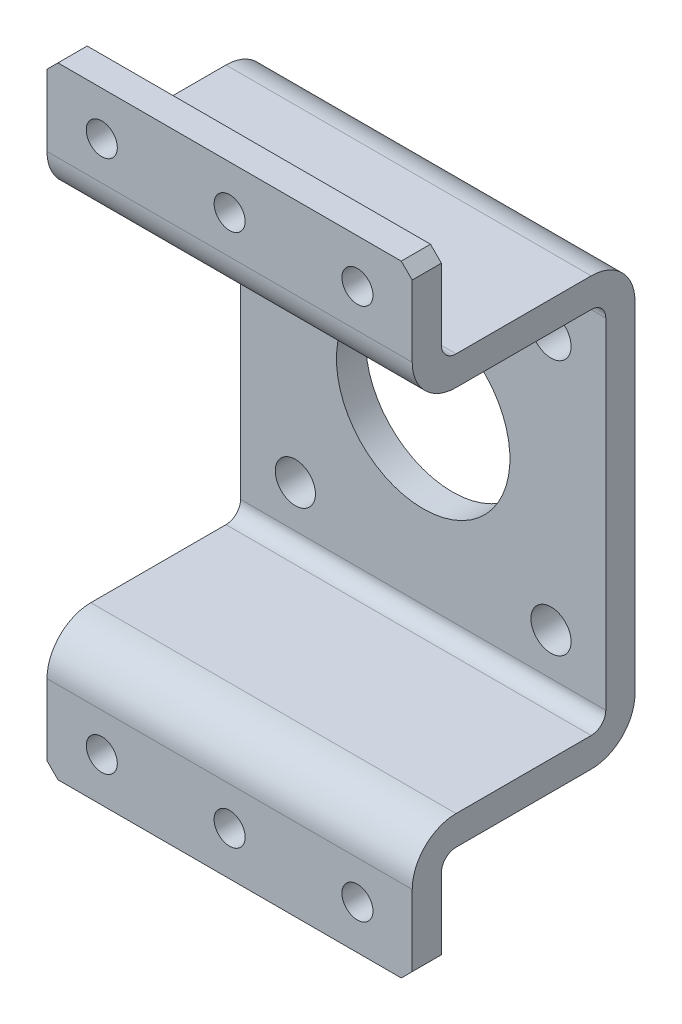
SolidWorks part; units mm, degrees
ref_plane "前视基准面" through (0, 0, 0) normal (0, 0, 1) x (1, 0, 0)
ref_plane "上视基准面" through (0, 0, 0) normal (0, 1, 0) x (1, 0, 0)
ref_plane "右视基准面" through (0, 0, 0) normal (1, 0, 0) x (0, 0, -1)
sketch "草图1" plane through (0, 0, 0) normal (1, 0, 0) x (0, 0, -1)
  line L0 (-61, 85) -> (-61, 50.5)
  line L1 (-53, 85) -> (-53, 58.5)
  line L2 (-53, 58.5) -> (0, 58.5)
  line L3 (0, 58.5) -> (0, -58.5)
  line L4 (0, -58.5) -> (-53, -58.5)
  line L5 (-53, -58.5) -> (-53, -85)
  line L6 (-61, 50.5) -> (-8, 50.5)
  line L7 (-8, 50.5) -> (-8, -50.5)
  line L8 (-8, -50.5) -> (-61, -50.5)
  line L9 (-61, -50.5) -> (-61, -85)
  line L10 (-61, 85) -> (-53, 85)
  line L11 (-61, -85) -> (-53, -85)
  line L12 (0, 0) -> (-67.8043, 0) construction
  point P2 (0, 0)
  dimension "D1" = 8
  dimension "D2" = 61
  dimension "D3" = 117
  dimension "D4" = 170
extrude "凸台-拉伸1" add sketch "草图1" along normal mid plane 100
sketch "草图3" plane through (0, 0, 0) normal (0, 0, -1) x (-1, 0, 0)
  circle A0 centre (0, 0) radius 23.75
  dimension "D1" = 47.5
extrude "切除-拉伸1" cut sketch "草图3" against normal through all
hole_wizard "Ø11.0 (11) 直径孔1" positions "草图5" profile "草图4" hole size "Ø11.0" standard "ISO" end condition through all
sketch "草图5" plane through (0, 0, 0) normal (0, 0, -1) x (-1, 0, 0)
  line L1 (-35, 35) -> (35, 35) construction
  line L2 (-35, 35) -> (-35, -35) construction
  line L3 (-35, -35) -> (35, -35) construction
  line L4 (35, 35) -> (35, -35) construction
  line L5 (-35, 35) -> (35, -35) construction
  line L6 (-35, -35) -> (35, 35) construction
  point P1 (0, 0)
  point P2 (35, -35)
  point P61 (-35, 35)
  point P62 (-35, -35)
  point P63 (35, 35)
  dimension "D1" = 70
  dimension "D2" = 70
sketch "草图4" plane through (0, 0, 0) normal (1, 0, 0) x (0, 1, 0)
  line L0 (0, 0) -> (0, 61)
  line L1 (0, 61) -> (5.5, 61)
  line L2 (5.5, 61) -> (5.5, 0)
  line L5 (5.5, 0) -> (0, 0)
  line L11 (0, -6.35) -> (0, 107.95) construction
  dimension "通孔孔直径" = 11
  dimension "通孔孔深度" = 61
hole_wizard "Ø8.5 (8.5) 直径孔1" positions "草图7" profile "草图6" hole size "Ø8.5" standard "ISO" end condition through all
sketch "草图7" plane through (0, 0, 53) normal (0, 0, -1) x (-1, 0, 0)
  line L0 (-50, -85) -> (50, -85) construction
  line L1 (-61.1344, 0) -> (74.3765, 0) construction
  point P0 (-35, -73)
  point P2 (0, -73)
  point P4 (35, -73)
  point P14 (35, 73)
  point P15 (0, 73)
  point P16 (-35, 73)
  dimension "D1" = 12
  dimension "D2" = 70
  dimension "D3" = 35
sketch "草图6" plane through (35, -73, 53) normal (1, 0, 0) x (0, 1, 0)
  line L0 (0, 0) -> (0, 8)
  line L1 (0, 8) -> (4.25, 8)
  line L2 (4.25, 8) -> (4.25, 0)
  line L5 (4.25, 0) -> (0, 0)
  line L11 (0, -6.35) -> (0, 107.95) construction
  dimension "通孔孔直径" = 8.5
  dimension "通孔孔深度" = 8
chamfer "倒角1" distance 3 angle 45 4 edges at (-50, 85, 57) (50, 85, 57) (-50, -85, 57) (50, -85, 57)
fillet "圆角1" radius 4 4 edges at (0, -58.5, 53) (0, 58.5, 53) (0, 50.5, 8) (0, -50.5, 8)
fillet "圆角2" radius 12 4 edges at (0, -58.5, 0) (0, 58.5, 0) (0, 50.5, 61) (0, -50.5, 61)
